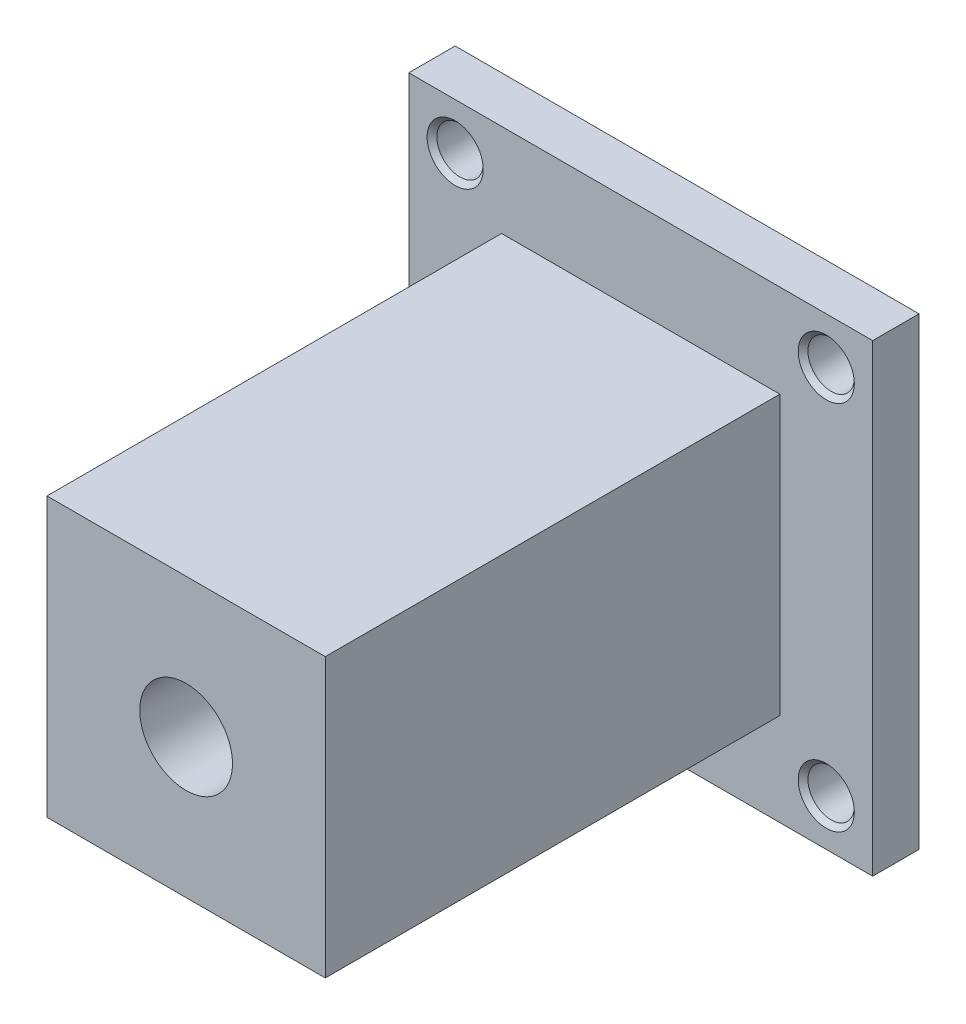
SolidWorks part; units mm, degrees
ref_plane "前视基准面" through (0, 0, 0) normal (0, 0, 1) x (1, 0, 0)
ref_plane "上视基准面" through (0, 0, 0) normal (0, 1, 0) x (1, 0, 0)
ref_plane "右视基准面" through (0, 0, 0) normal (1, 0, 0) x (0, 0, -1)
sketch "草图1" plane through (0, 0, 0) normal (0, 0, 1) x (1, 0, 0)
  line L0 (0, 0) -> (-50, 0) construction
  line L2 (-35, 15) -> (-65, 15)
  line L3 (-35, 15) -> (-35, -15)
  line L4 (-35, -15) -> (-65, -15)
  line L5 (-65, 15) -> (-65, -15)
  line L6 (-35, 15) -> (-65, -15) construction
  line L7 (-35, -15) -> (-65, 15) construction
  dimension "D1" = 30
  dimension "D2" = 50
extrude "凸台-拉伸1" add sketch "草图1" along normal blind 54
sketch "草图2" plane through (0, 0, 0) normal (0, 0, 1) x (1, 0, 0)
  line L8 (-75, 25) -> (-75, -25)
  line L9 (-75, -25) -> (-25, -25)
  line L10 (-25, -25) -> (-25, 25)
  line L11 (-25, 25) -> (-75, 25)
  line L12 (-75, 25) -> (-75, -25)
  line L13 (-75, -25) -> (-25, -25)
  line L14 (-25, -25) -> (-25, 25)
  line L15 (-25, 25) -> (-75, 25)
  dimension "D1" = 10
extrude "凸台-拉伸2" add sketch "草图2" along normal blind 5
sketch "草图3" plane through (0, 0, 5) normal (0, 0, 1) x (1, 0, 0)
  line L8 (-30, 20) -> (-70, 20)
  line L9 (-70, 20) -> (-70, -20)
  line L10 (-70, -20) -> (-30, -20)
  line L11 (-30, -20) -> (-30, 20)
  line L12 (-30, 20) -> (-70, 20)
  line L13 (-70, 20) -> (-70, -20)
  line L14 (-70, -20) -> (-30, -20)
  line L15 (-30, -20) -> (-30, 20)
  dimension "D1" = 5
hole_wizard "M6 螺纹孔1" positions "草图4" profile "草图5" tap size "M6" standard "GB"
sketch "草图4" plane through (0, 0, 5) normal (0, 0, 1) x (1, 0, 0)
  point P0 (-30, 20)
  point P3 (-70, 20)
  point P6 (-70, -20)
  point P9 (-30, -20)
sketch "草图5" plane through (-30, 20, 5) normal (1, 0, 0) x (0, -1, 0)
  line L0 (0, 0) -> (0, 15)
  line L1 (0, 15) -> (2.5, 13.4978)
  line L2 (2.5, 13.4978) -> (2.5, 0.525)
  line L3 (2.5, 0.525) -> (3.025, 0)
  line L5 (3.025, 0) -> (0, 0)
  line L6 (-2.5, 0.525) -> (-3.025, 0) construction
  line L10 (0, 15) -> (-2.5, 13.4978) construction
  line L11 (0, -6.35) -> (0, 107.95) construction
  dimension "螺纹孔钻头直径" = 5
  dimension "螺纹孔钻头深度" = 15
  dimension "近端锥形沉头孔直径" = 6.05
  dimension "近端锥形沉头孔角度" = 90
  dimension "导头角度" = 118
cosmetic thread "孔螺蚊线1" parameters "D1"=12, "D2"=6
cosmetic thread "孔螺蚊线2" parameters "D1"=12, "D2"=6
cosmetic thread "孔螺蚊线3" parameters "D1"=12, "D2"=6
cosmetic thread "孔螺蚊线4" parameters "D1"=12, "D2"=6
sketch "草图6" plane through (0, 0, 54) normal (0, 0, 1) x (1, 0, 0)
  line L0 (-65, 15) -> (-35, -15) construction
  circle A0 centre (-50, 0) radius 5
  dimension "D1" = 10
extrude "切除-拉伸1" cut sketch "草图6" against normal blind 39
